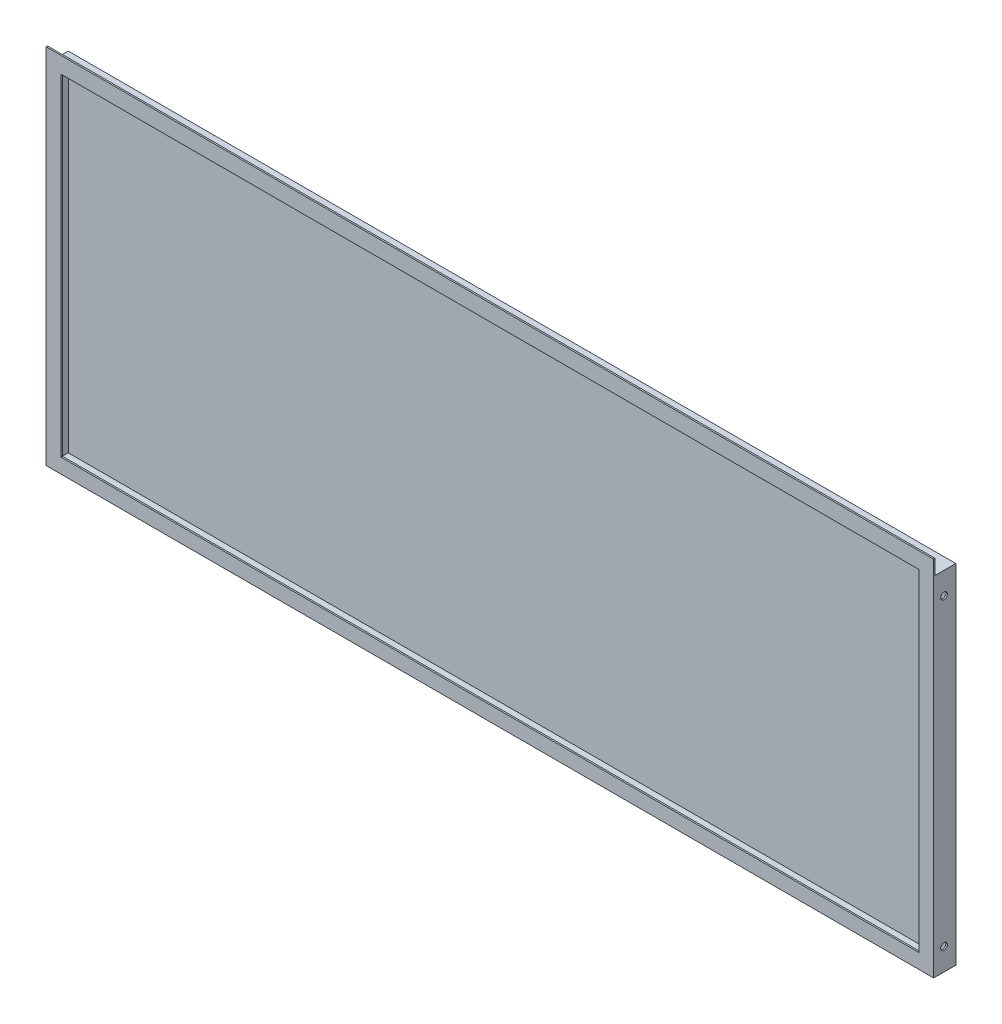
from build123d import *

# Parameters (mm, degrees)
SKETCH_1_W               = 1204
SKETCH_1_H               = 472
EXTRUDE_1_DEPTH          = 30
SHELL_1_T                = -2
SKETCH_2_W               = 1204
SKETCH_2_H               = 492
SKETCH_2_W_2             = 1164
SKETCH_2_H_2             = 450
EXTRUDE_2_DEPTH          = 2
CUT_EXTRUDE_1_DEPTH      = 1295
CUT_EXTRUDE_1_DEPTH_BACK = 72
SKETCH_3_R               = 4.5
SKETCH_4_R               = 4.5
CUT_EXTRUDE_2_DEPTH      = 45


with BuildPart() as part:
    # 草图1 → 凸台-拉伸1 (new body)
    with BuildSketch(Plane.XY):
        with Locations((602, 236)):
            Rectangle(SKETCH_1_W, SKETCH_1_H)
    extrude(amount=EXTRUDE_1_DEPTH)

    # 抽壳1
    shell_1_openings = [part.faces().sort_by_distance(p)[0] for p in [
        (602, 236, 30),
    ]]
    offset(amount=SHELL_1_T, openings=shell_1_openings, kind=Kind.INTERSECTION)

    # 草图2 → 凸台-拉伸2 (add)
    with BuildSketch(Plane.XY.offset(30)):
        with Locations((602, 246)):
            Rectangle(SKETCH_2_W, SKETCH_2_H)
        with Locations((602, 245)):
            Rectangle(SKETCH_2_W_2, SKETCH_2_H_2, mode=Mode.SUBTRACT)
    extrude(amount=-EXTRUDE_2_DEPTH)

    # 草图3 → 切除-拉伸1 (cut, two sides: drawn at the far end of the back side and taken through both)
    with BuildSketch(Plane(origin=(2, 0, 0), x_dir=(0, 0, -1), z_dir=(1, 0, 0)).offset(-CUT_EXTRUDE_1_DEPTH_BACK)):
        with Locations(Location((-16, 442, 0), (0, 0, 180))):
            Circle(SKETCH_3_R)
        with Locations(Location((-16, 30, 0), (0, 0, 180))):
            Circle(SKETCH_3_R)
    extrude(amount=CUT_EXTRUDE_1_DEPTH + CUT_EXTRUDE_1_DEPTH_BACK, mode=Mode.SUBTRACT)

    # 草图4 → 切除-拉伸2 (cut)
    with BuildSketch(Plane(origin=(0, 2, 0), x_dir=(1, 0, 0), z_dir=(0, 1, 0))):
        with Locations(Location((1174, -16, 0), (0, 0, 270))):
            Circle(SKETCH_4_R)
        with Locations(Location((30, -16, 0), (0, 0, 270))):
            Circle(SKETCH_4_R)
        with Locations(Location((1065, -16, 0), (0, 0, 270))):
            Circle(SKETCH_4_R)
        with Locations(Location((965, -16, 0), (0, 0, 270))):
            Circle(SKETCH_4_R)
        with Locations(Location((500, -16, 0), (0, 0, 270))):
            Circle(SKETCH_4_R)
    extrude(amount=-CUT_EXTRUDE_2_DEPTH, mode=Mode.SUBTRACT)


solid = part.part
